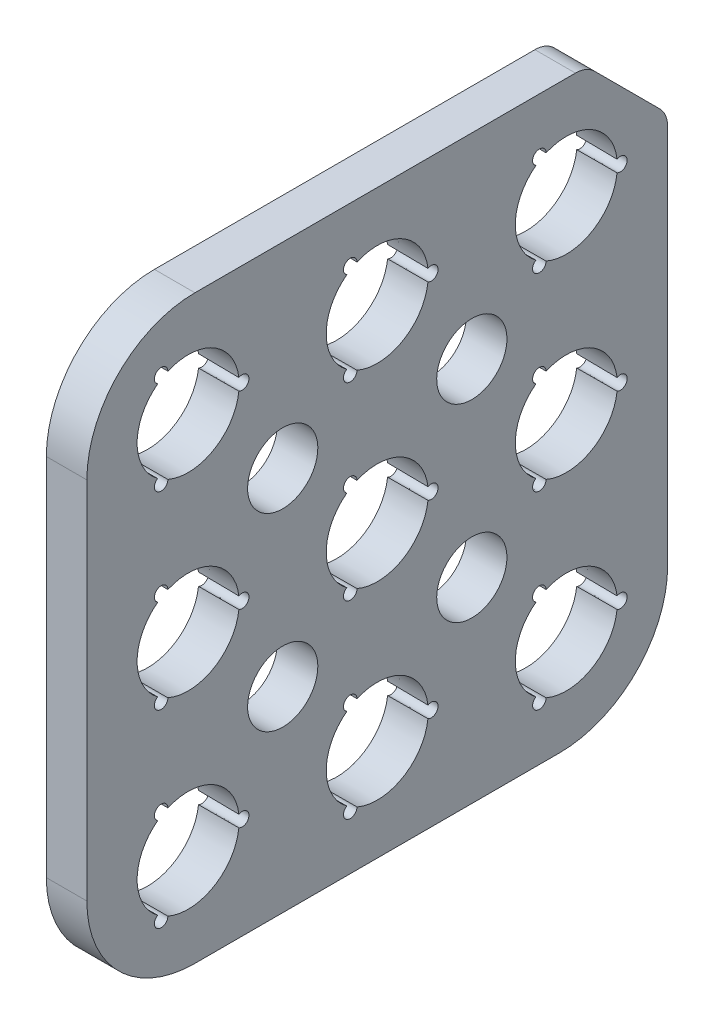
from build123d import *

# Parameters (mm, degrees)
SKETCH_1_W                        = 230
SKETCH_1_H                        = 230
EXTRUDE_1_DEPTH                   = 12.5
SKETCH_6_R                        = 2.475
CUT_EXTRUDE_1_DEPTH               = 47
CUT_EXTRUDE_1_DRAFT               = -0.3
CUT_EXTRUDE_1_PROFILE_2_DEPTH     = 47
CUT_EXTRUDE_1_PROFILE_2_DRAFT     = -0.3
CUT_EXTRUDE_1_PROFILE_3_DEPTH     = 47
CUT_EXTRUDE_1_PROFILE_3_DRAFT     = -0.3
CUT_EXTRUDE_2_DEPTH               = 4
PATTERN_LINEAR_3_COUNT            = 3
PATTERN_LINEAR_3_PITCH            = 70
PATTERN_LINEAR_3_COUNT_DIR2       = 3
PATTERN_LINEAR_3_PITCH_DIR2       = 70
PATTERN_LINEAR_3_COPY_1_SKETCH_R  = 2.475
PATTERN_LINEAR_3_COPY_1_DEPTH     = 47
PATTERN_LINEAR_3_COPY_1_DRAFT     = -0.3
PATTERN_LINEAR_3_COPY_2_SKETCH_R  = 2.475
PATTERN_LINEAR_3_COPY_2_DEPTH     = 47
PATTERN_LINEAR_3_COPY_2_DRAFT     = -0.3
PATTERN_LINEAR_3_COPY_3_SKETCH_R  = 2.475
PATTERN_LINEAR_3_COPY_3_DEPTH     = 47
PATTERN_LINEAR_3_COPY_3_DRAFT     = -0.3
PATTERN_LINEAR_3_COPY_4_SKETCH_R  = 2.475
PATTERN_LINEAR_3_COPY_4_DEPTH     = 47
PATTERN_LINEAR_3_COPY_4_DRAFT     = -0.3
PATTERN_LINEAR_3_COPY_5_SKETCH_R  = 2.475
PATTERN_LINEAR_3_COPY_5_DEPTH     = 47
PATTERN_LINEAR_3_COPY_5_DRAFT     = -0.3
PATTERN_LINEAR_3_COPY_6_SKETCH_R  = 2.475
PATTERN_LINEAR_3_COPY_6_DEPTH     = 47
PATTERN_LINEAR_3_COPY_6_DRAFT     = -0.3
PATTERN_LINEAR_3_COPY_7_SKETCH_R  = 2.475
PATTERN_LINEAR_3_COPY_7_DEPTH     = 47
PATTERN_LINEAR_3_COPY_7_DRAFT     = -0.3
PATTERN_LINEAR_3_COPY_8_SKETCH_R  = 2.475
PATTERN_LINEAR_3_COPY_8_DEPTH     = 47
PATTERN_LINEAR_3_COPY_8_DRAFT     = -0.3
PATTERN_LINEAR_3_COPY_9_SKETCH_R  = 2.475
PATTERN_LINEAR_3_COPY_9_DEPTH     = 47
PATTERN_LINEAR_3_COPY_9_DRAFT     = -0.3
PATTERN_LINEAR_3_COPY_10_SKETCH_R = 2.475
PATTERN_LINEAR_3_COPY_10_DEPTH    = 47
PATTERN_LINEAR_3_COPY_10_DRAFT    = -0.3
PATTERN_LINEAR_3_COPY_11_SKETCH_R = 2.475
PATTERN_LINEAR_3_COPY_11_DEPTH    = 47
PATTERN_LINEAR_3_COPY_11_DRAFT    = -0.3
PATTERN_LINEAR_3_COPY_12_SKETCH_R = 2.475
PATTERN_LINEAR_3_COPY_12_DEPTH    = 47
PATTERN_LINEAR_3_COPY_12_DRAFT    = -0.3
PATTERN_LINEAR_3_COPY_13_SKETCH_R = 2.475
PATTERN_LINEAR_3_COPY_13_DEPTH    = 47
PATTERN_LINEAR_3_COPY_13_DRAFT    = -0.3
PATTERN_LINEAR_3_COPY_14_SKETCH_R = 2.475
PATTERN_LINEAR_3_COPY_14_DEPTH    = 47
PATTERN_LINEAR_3_COPY_14_DRAFT    = -0.3
PATTERN_LINEAR_3_COPY_15_SKETCH_R = 2.475
PATTERN_LINEAR_3_COPY_15_DEPTH    = 47
PATTERN_LINEAR_3_COPY_15_DRAFT    = -0.3
PATTERN_LINEAR_3_COPY_16_SKETCH_R = 2.475
PATTERN_LINEAR_3_COPY_16_DEPTH    = 47
PATTERN_LINEAR_3_COPY_16_DRAFT    = -0.3
PATTERN_LINEAR_3_COPY_17_SKETCH_R = 2.475
PATTERN_LINEAR_3_COPY_17_DEPTH    = 47
PATTERN_LINEAR_3_COPY_17_DRAFT    = -0.3
PATTERN_LINEAR_3_COPY_18_SKETCH_R = 2.475
PATTERN_LINEAR_3_COPY_18_DEPTH    = 47
PATTERN_LINEAR_3_COPY_18_DRAFT    = -0.3
PATTERN_LINEAR_3_COPY_19_SKETCH_R = 2.475
PATTERN_LINEAR_3_COPY_19_DEPTH    = 47
PATTERN_LINEAR_3_COPY_19_DRAFT    = -0.3
PATTERN_LINEAR_3_COPY_20_SKETCH_R = 2.475
PATTERN_LINEAR_3_COPY_20_DEPTH    = 47
PATTERN_LINEAR_3_COPY_20_DRAFT    = -0.3
PATTERN_LINEAR_3_COPY_21_SKETCH_R = 2.475
PATTERN_LINEAR_3_COPY_21_DEPTH    = 47
PATTERN_LINEAR_3_COPY_21_DRAFT    = -0.3
PATTERN_LINEAR_3_COPY_22_SKETCH_R = 2.475
PATTERN_LINEAR_3_COPY_22_DEPTH    = 47
PATTERN_LINEAR_3_COPY_22_DRAFT    = -0.3
PATTERN_LINEAR_3_COPY_23_SKETCH_R = 2.475
PATTERN_LINEAR_3_COPY_23_DEPTH    = 47
PATTERN_LINEAR_3_COPY_23_DRAFT    = -0.3
PATTERN_LINEAR_3_COPY_24_SKETCH_R = 2.475
PATTERN_LINEAR_3_COPY_24_DEPTH    = 47
PATTERN_LINEAR_3_COPY_24_DRAFT    = -0.3
PATTERN_LINEAR_3_COPY_25_SKETCH_R = 2.475
PATTERN_LINEAR_3_COPY_25_DEPTH    = 47
PATTERN_LINEAR_3_COPY_25_DRAFT    = -0.3
PATTERN_LINEAR_3_COPY_26_SKETCH_R = 2.475
PATTERN_LINEAR_3_COPY_26_DEPTH    = 47
PATTERN_LINEAR_3_COPY_26_DRAFT    = -0.3
PATTERN_LINEAR_3_COPY_27_SKETCH_R = 2.475
PATTERN_LINEAR_3_COPY_27_DEPTH    = 47
PATTERN_LINEAR_3_COPY_27_DRAFT    = -0.3
PATTERN_LINEAR_3_COPY_28_SKETCH_R = 2.475
PATTERN_LINEAR_3_COPY_28_DEPTH    = 47
PATTERN_LINEAR_3_COPY_28_DRAFT    = -0.3
PATTERN_LINEAR_3_COPY_29_SKETCH_R = 2.475
PATTERN_LINEAR_3_COPY_29_DEPTH    = 47
PATTERN_LINEAR_3_COPY_29_DRAFT    = -0.3
PATTERN_LINEAR_3_COPY_30_SKETCH_R = 2.475
PATTERN_LINEAR_3_COPY_30_DEPTH    = 47
PATTERN_LINEAR_3_COPY_30_DRAFT    = -0.3
PATTERN_LINEAR_3_COPY_31_SKETCH_R = 2.475
PATTERN_LINEAR_3_COPY_31_DEPTH    = 47
PATTERN_LINEAR_3_COPY_31_DRAFT    = -0.3
PATTERN_LINEAR_3_COPY_32_SKETCH_R = 2.475
PATTERN_LINEAR_3_COPY_32_DEPTH    = 47
PATTERN_LINEAR_3_COPY_32_DRAFT    = -0.3
PATTERN_LINEAR_3_COPY_33_SKETCH_R = 2.475
PATTERN_LINEAR_3_COPY_33_DEPTH    = 47
PATTERN_LINEAR_3_COPY_33_DRAFT    = -0.3
PATTERN_LINEAR_3_COPY_34_SKETCH_R = 2.475
PATTERN_LINEAR_3_COPY_34_DEPTH    = 47
PATTERN_LINEAR_3_COPY_34_DRAFT    = -0.3
PATTERN_LINEAR_3_COPY_35_SKETCH_R = 2.475
PATTERN_LINEAR_3_COPY_35_DEPTH    = 47
PATTERN_LINEAR_3_COPY_35_DRAFT    = -0.3
PATTERN_LINEAR_3_COPY_36_SKETCH_R = 2.475
PATTERN_LINEAR_3_COPY_36_DEPTH    = 47
PATTERN_LINEAR_3_COPY_36_DRAFT    = -0.3
PATTERN_LINEAR_3_COPY_37_SKETCH_R = 2.475
PATTERN_LINEAR_3_COPY_37_DEPTH    = 47
PATTERN_LINEAR_3_COPY_37_DRAFT    = -0.3
PATTERN_LINEAR_3_COPY_38_SKETCH_R = 2.475
PATTERN_LINEAR_3_COPY_38_DEPTH    = 47
PATTERN_LINEAR_3_COPY_38_DRAFT    = -0.3
PATTERN_LINEAR_3_COPY_39_SKETCH_R = 2.475
PATTERN_LINEAR_3_COPY_39_DEPTH    = 47
PATTERN_LINEAR_3_COPY_39_DRAFT    = -0.3
PATTERN_LINEAR_3_COPY_40_SKETCH_R = 2.475
PATTERN_LINEAR_3_COPY_40_DEPTH    = 47
PATTERN_LINEAR_3_COPY_40_DRAFT    = -0.3
SKETCH_8_W                        = 34.590931249
SKETCH_8_H                        = 260.535950259
CUT_EXTRUDE_3_DEPTH               = 626
SKETCH_9_W                        = 249.849241437
SKETCH_9_H                        = 239.022710494
CUT_EXTRUDE_4_DEPTH               = 626
SKETCH_10_W                       = 30.276924454
SKETCH_10_H                       = 249.230780566
CUT_EXTRUDE_5_DEPTH               = 313
SKETCH_11_W                       = 446.10197795
SKETCH_11_H                       = 340.76642687
SKETCH_11_W_2                     = 215
SKETCH_11_H_2                     = 215
CUT_EXTRUDE_6_DEPTH               = 120
CHAMFER_1_SIZE                    = 30
FILLET_1_R                        = 10
FILLET_2_R                        = 40
SKETCH_14_R                       = 13
CUT_EXTRUDE_7_DEPTH               = 120
PATTERN_LINEAR_6_COUNT            = 2
PATTERN_LINEAR_6_PITCH            = 70
PATTERN_LINEAR_6_COUNT_DIR2       = 2
PATTERN_LINEAR_6_PITCH_DIR2       = 70


with BuildPart() as part:
    # 草图1 → 凸台-拉伸1 (new, symmetric)
    with BuildSketch(Plane(origin=(0, 0, 0), x_dir=(0, 0, -1), z_dir=(1, 0, 0))):
        Rectangle(SKETCH_1_W, SKETCH_1_H)
    extrude(amount=EXTRUDE_1_DEPTH, both=True)

    # 草图5 → 切除-旋转1 (revolve, cut)
    with BuildSketch(Plane(origin=(0, 70, 0), x_dir=(1, 0, 0), z_dir=(0, 1, 0))):
        Polygon((9.1, 70), (9.1, 88.87), (-16.76003836, 89.005404082), (-16.76003836, 70), align=None)
    cut_revolve_1 = revolve(axis=Axis((12.711537601, 70, -70), (-1, 0, 0)), mode=Mode.SUBTRACT)


with BuildPart() as cut_extrude_1_tool:
    # 草图6 → 切除-拉伸1 (with draft: the straight prism first)
    with BuildSketch(Plane.ZY.offset(-9.1)):
        with Locations((-60, 87.320508076)):
            Circle(SKETCH_6_R)
    extrude(amount=CUT_EXTRUDE_1_DEPTH)
    # 切除-拉伸1: the draft: its side faces are tilted about the plane it starts from
    cut_extrude_1_sides = [cut_extrude_1_tool.faces().sort_by_distance(p)[0] for p in [
        (-14.4, 87.320508076, -62.475),
    ]]
    draft(cut_extrude_1_sides, Plane.ZY.offset(-9.1), CUT_EXTRUDE_1_DRAFT)


with BuildPart() as part_1:
    add(part.part)

    # 切除-拉伸1: cut by cut_extrude_1_tool
    add(cut_extrude_1_tool.part, mode=Mode.SUBTRACT)


with BuildPart() as cut_extrude_1_profile_2_tool:
    # 草图6 → 切除-拉伸1 profile 2 (with draft: the straight prism first)
    with BuildSketch(Plane.ZY.offset(-9.1)):
        with Locations((-60, 52.679491924)):
            Circle(SKETCH_6_R)
    extrude(amount=CUT_EXTRUDE_1_PROFILE_2_DEPTH)
    # 切除-拉伸1 profile 2: the draft: its side faces are tilted about the plane it starts from
    cut_extrude_1_profile_2_sides = [cut_extrude_1_profile_2_tool.faces().sort_by_distance(p)[0] for p in [
        (-14.4, 52.679491924, -62.475),
    ]]
    draft(cut_extrude_1_profile_2_sides, Plane.ZY.offset(-9.1), CUT_EXTRUDE_1_PROFILE_2_DRAFT)


with BuildPart() as part_2:
    add(part_1.part)

    # 切除-拉伸1 profile 2: cut by cut_extrude_1_profile_2_tool
    add(cut_extrude_1_profile_2_tool.part, mode=Mode.SUBTRACT)


with BuildPart() as cut_extrude_1_profile_3_tool:
    # 草图6 → 切除-拉伸1 profile 3 (with draft: the straight prism first)
    with BuildSketch(Plane.ZY.offset(-9.1)):
        with Locations((-90, 70)):
            Circle(SKETCH_6_R)
    extrude(amount=CUT_EXTRUDE_1_PROFILE_3_DEPTH)
    # 切除-拉伸1 profile 3: the draft: its side faces are tilted about the plane it starts from
    cut_extrude_1_profile_3_sides = [cut_extrude_1_profile_3_tool.faces().sort_by_distance(p)[0] for p in [
        (-14.4, 70, -92.475),
    ]]
    draft(cut_extrude_1_profile_3_sides, Plane.ZY.offset(-9.1), CUT_EXTRUDE_1_PROFILE_3_DRAFT)


with BuildPart() as part_3:
    add(part_2.part)

    # 切除-拉伸1 profile 3: cut by cut_extrude_1_profile_3_tool
    add(cut_extrude_1_profile_3_tool.part, mode=Mode.SUBTRACT)

    # 草图7 → 切除-拉伸2 (cut)
    with BuildSketch(Plane.ZY.offset(12.5)):
        with BuildLine():
            Line((-80.578681475, 81.195601737), (-84.104368777, 87.242876251))
            ThreePointArc((-84.104368777, 87.242876251), (-82.843575171, 92.029357159), (-78.057094263, 90.768563553))
            Line((-78.057094263, 90.768563553), (-74.531406961, 84.721289038))
            ThreePointArc((-74.531406961, 84.721289038), (-75.792200567, 79.934808131), (-80.578681475, 81.195601737))
        make_face()
        with BuildLine():
            Line((-73.5, 85), (-73.5, 92))
            ThreePointArc((-73.5, 92), (-70, 95.5), (-66.5, 92))
            Line((-66.5, 92), (-66.5, 85))
            ThreePointArc((-66.5, 85), (-70, 81.5), (-73.5, 85))
        make_face()
    cut_extrude_2 = extrude(amount=-CUT_EXTRUDE_2_DEPTH, mode=Mode.SUBTRACT)

    # 阵列(线性)3: 切除-旋转1, Cut-Extrude 2 3 × 3
    with Locations(*[(0, -j * PATTERN_LINEAR_3_PITCH_DIR2, i * PATTERN_LINEAR_3_PITCH) for i in range(PATTERN_LINEAR_3_COUNT) for j in range(PATTERN_LINEAR_3_COUNT_DIR2) if (i, j) != (0, 0)]):
        add(cut_revolve_1, mode=Mode.SUBTRACT)
        add(cut_extrude_2, mode=Mode.SUBTRACT)


with BuildPart() as pattern_linear_3_copy_1_tool:
    # 阵列(线性)3 copy 1 sketch → 阵列(线性)3 copy 1 (with draft: the straight prism first)
    with BuildSketch(Plane(origin=(9.1, -70, 0), x_dir=(0, 0, 1), z_dir=(-1, 0, 0))):
        with Locations((-60, 87.320508076)):
            Circle(PATTERN_LINEAR_3_COPY_1_SKETCH_R)
    extrude(amount=PATTERN_LINEAR_3_COPY_1_DEPTH)
    # 阵列(线性)3 copy 1: the draft: its side faces are tilted about the plane it starts from
    pattern_linear_3_copy_1_sides = [pattern_linear_3_copy_1_tool.faces().sort_by_distance(p)[0] for p in [
        (-14.4, 17.320508076, -62.475),
    ]]
    draft(pattern_linear_3_copy_1_sides, Plane(origin=(9.1, -70, 0), x_dir=(0, 0, 1), z_dir=(-1, 0, 0)), PATTERN_LINEAR_3_COPY_1_DRAFT)


with BuildPart() as part_4:
    add(part_3.part)

    # 阵列(线性)3 copy 1: cut by pattern_linear_3_copy_1_tool
    add(pattern_linear_3_copy_1_tool.part, mode=Mode.SUBTRACT)


with BuildPart() as pattern_linear_3_copy_2_tool:
    # 阵列(线性)3 copy 2 sketch → 阵列(线性)3 copy 2 (with draft: the straight prism first)
    with BuildSketch(Plane(origin=(9.1, -140, 0), x_dir=(0, 0, 1), z_dir=(-1, 0, 0))):
        with Locations((-60, 87.320508076)):
            Circle(PATTERN_LINEAR_3_COPY_2_SKETCH_R)
    extrude(amount=PATTERN_LINEAR_3_COPY_2_DEPTH)
    # 阵列(线性)3 copy 2: the draft: its side faces are tilted about the plane it starts from
    pattern_linear_3_copy_2_sides = [pattern_linear_3_copy_2_tool.faces().sort_by_distance(p)[0] for p in [
        (-14.4, -52.679491924, -62.475),
    ]]
    draft(pattern_linear_3_copy_2_sides, Plane(origin=(9.1, -140, 0), x_dir=(0, 0, 1), z_dir=(-1, 0, 0)), PATTERN_LINEAR_3_COPY_2_DRAFT)


with BuildPart() as part_5:
    add(part_4.part)

    # 阵列(线性)3 copy 2: cut by pattern_linear_3_copy_2_tool
    add(pattern_linear_3_copy_2_tool.part, mode=Mode.SUBTRACT)


with BuildPart() as pattern_linear_3_copy_3_tool:
    # 阵列(线性)3 copy 3 sketch → 阵列(线性)3 copy 3 (with draft: the straight prism first)
    with BuildSketch(Plane(origin=(9.1, 0, 70), x_dir=(0, 0, 1), z_dir=(-1, 0, 0))):
        with Locations((-60, 87.320508076)):
            Circle(PATTERN_LINEAR_3_COPY_3_SKETCH_R)
    extrude(amount=PATTERN_LINEAR_3_COPY_3_DEPTH)
    # 阵列(线性)3 copy 3: the draft: its side faces are tilted about the plane it starts from
    pattern_linear_3_copy_3_sides = [pattern_linear_3_copy_3_tool.faces().sort_by_distance(p)[0] for p in [
        (-14.4, 87.320508076, 7.525),
    ]]
    draft(pattern_linear_3_copy_3_sides, Plane(origin=(9.1, 0, 70), x_dir=(0, 0, 1), z_dir=(-1, 0, 0)), PATTERN_LINEAR_3_COPY_3_DRAFT)


with BuildPart() as part_6:
    add(part_5.part)

    # 阵列(线性)3 copy 3: cut by pattern_linear_3_copy_3_tool
    add(pattern_linear_3_copy_3_tool.part, mode=Mode.SUBTRACT)


with BuildPart() as pattern_linear_3_copy_4_tool:
    # 阵列(线性)3 copy 4 sketch → 阵列(线性)3 copy 4 (with draft: the straight prism first)
    with BuildSketch(Plane(origin=(9.1, -70, 70), x_dir=(0, 0, 1), z_dir=(-1, 0, 0))):
        with Locations((-60, 87.320508076)):
            Circle(PATTERN_LINEAR_3_COPY_4_SKETCH_R)
    extrude(amount=PATTERN_LINEAR_3_COPY_4_DEPTH)
    # 阵列(线性)3 copy 4: the draft: its side faces are tilted about the plane it starts from
    pattern_linear_3_copy_4_sides = [pattern_linear_3_copy_4_tool.faces().sort_by_distance(p)[0] for p in [
        (-14.4, 17.320508076, 7.525),
    ]]
    draft(pattern_linear_3_copy_4_sides, Plane(origin=(9.1, -70, 70), x_dir=(0, 0, 1), z_dir=(-1, 0, 0)), PATTERN_LINEAR_3_COPY_4_DRAFT)


with BuildPart() as part_7:
    add(part_6.part)

    # 阵列(线性)3 copy 4: cut by pattern_linear_3_copy_4_tool
    add(pattern_linear_3_copy_4_tool.part, mode=Mode.SUBTRACT)


with BuildPart() as pattern_linear_3_copy_5_tool:
    # 阵列(线性)3 copy 5 sketch → 阵列(线性)3 copy 5 (with draft: the straight prism first)
    with BuildSketch(Plane(origin=(9.1, -140, 70), x_dir=(0, 0, 1), z_dir=(-1, 0, 0))):
        with Locations((-60, 87.320508076)):
            Circle(PATTERN_LINEAR_3_COPY_5_SKETCH_R)
    extrude(amount=PATTERN_LINEAR_3_COPY_5_DEPTH)
    # 阵列(线性)3 copy 5: the draft: its side faces are tilted about the plane it starts from
    pattern_linear_3_copy_5_sides = [pattern_linear_3_copy_5_tool.faces().sort_by_distance(p)[0] for p in [
        (-14.4, -52.679491924, 7.525),
    ]]
    draft(pattern_linear_3_copy_5_sides, Plane(origin=(9.1, -140, 70), x_dir=(0, 0, 1), z_dir=(-1, 0, 0)), PATTERN_LINEAR_3_COPY_5_DRAFT)


with BuildPart() as part_8:
    add(part_7.part)

    # 阵列(线性)3 copy 5: cut by pattern_linear_3_copy_5_tool
    add(pattern_linear_3_copy_5_tool.part, mode=Mode.SUBTRACT)


with BuildPart() as pattern_linear_3_copy_6_tool:
    # 阵列(线性)3 copy 6 sketch → 阵列(线性)3 copy 6 (with draft: the straight prism first)
    with BuildSketch(Plane(origin=(9.1, 0, 140), x_dir=(0, 0, 1), z_dir=(-1, 0, 0))):
        with Locations((-60, 87.320508076)):
            Circle(PATTERN_LINEAR_3_COPY_6_SKETCH_R)
    extrude(amount=PATTERN_LINEAR_3_COPY_6_DEPTH)
    # 阵列(线性)3 copy 6: the draft: its side faces are tilted about the plane it starts from
    pattern_linear_3_copy_6_sides = [pattern_linear_3_copy_6_tool.faces().sort_by_distance(p)[0] for p in [
        (-14.4, 87.320508076, 77.525),
    ]]
    draft(pattern_linear_3_copy_6_sides, Plane(origin=(9.1, 0, 140), x_dir=(0, 0, 1), z_dir=(-1, 0, 0)), PATTERN_LINEAR_3_COPY_6_DRAFT)


with BuildPart() as part_9:
    add(part_8.part)

    # 阵列(线性)3 copy 6: cut by pattern_linear_3_copy_6_tool
    add(pattern_linear_3_copy_6_tool.part, mode=Mode.SUBTRACT)


with BuildPart() as pattern_linear_3_copy_7_tool:
    # 阵列(线性)3 copy 7 sketch → 阵列(线性)3 copy 7 (with draft: the straight prism first)
    with BuildSketch(Plane(origin=(9.1, -70, 140), x_dir=(0, 0, 1), z_dir=(-1, 0, 0))):
        with Locations((-60, 87.320508076)):
            Circle(PATTERN_LINEAR_3_COPY_7_SKETCH_R)
    extrude(amount=PATTERN_LINEAR_3_COPY_7_DEPTH)
    # 阵列(线性)3 copy 7: the draft: its side faces are tilted about the plane it starts from
    pattern_linear_3_copy_7_sides = [pattern_linear_3_copy_7_tool.faces().sort_by_distance(p)[0] for p in [
        (-14.4, 17.320508076, 77.525),
    ]]
    draft(pattern_linear_3_copy_7_sides, Plane(origin=(9.1, -70, 140), x_dir=(0, 0, 1), z_dir=(-1, 0, 0)), PATTERN_LINEAR_3_COPY_7_DRAFT)


with BuildPart() as part_10:
    add(part_9.part)

    # 阵列(线性)3 copy 7: cut by pattern_linear_3_copy_7_tool
    add(pattern_linear_3_copy_7_tool.part, mode=Mode.SUBTRACT)


with BuildPart() as pattern_linear_3_copy_8_tool:
    # 阵列(线性)3 copy 8 sketch → 阵列(线性)3 copy 8 (with draft: the straight prism first)
    with BuildSketch(Plane(origin=(9.1, -140, 140), x_dir=(0, 0, 1), z_dir=(-1, 0, 0))):
        with Locations((-60, 87.320508076)):
            Circle(PATTERN_LINEAR_3_COPY_8_SKETCH_R)
    extrude(amount=PATTERN_LINEAR_3_COPY_8_DEPTH)
    # 阵列(线性)3 copy 8: the draft: its side faces are tilted about the plane it starts from
    pattern_linear_3_copy_8_sides = [pattern_linear_3_copy_8_tool.faces().sort_by_distance(p)[0] for p in [
        (-14.4, -52.679491924, 77.525),
    ]]
    draft(pattern_linear_3_copy_8_sides, Plane(origin=(9.1, -140, 140), x_dir=(0, 0, 1), z_dir=(-1, 0, 0)), PATTERN_LINEAR_3_COPY_8_DRAFT)


with BuildPart() as part_11:
    add(part_10.part)

    # 阵列(线性)3 copy 8: cut by pattern_linear_3_copy_8_tool
    add(pattern_linear_3_copy_8_tool.part, mode=Mode.SUBTRACT)


with BuildPart() as pattern_linear_3_copy_9_tool:
    # 阵列(线性)3 copy 9 sketch → 阵列(线性)3 copy 9 (with draft: the straight prism first)
    with BuildSketch(Plane(origin=(9.1, -70, 0), x_dir=(0, 0, 1), z_dir=(-1, 0, 0))):
        with Locations((-60, 52.679491924)):
            Circle(PATTERN_LINEAR_3_COPY_9_SKETCH_R)
    extrude(amount=PATTERN_LINEAR_3_COPY_9_DEPTH)
    # 阵列(线性)3 copy 9: the draft: its side faces are tilted about the plane it starts from
    pattern_linear_3_copy_9_sides = [pattern_linear_3_copy_9_tool.faces().sort_by_distance(p)[0] for p in [
        (-14.4, -17.320508076, -62.475),
    ]]
    draft(pattern_linear_3_copy_9_sides, Plane(origin=(9.1, -70, 0), x_dir=(0, 0, 1), z_dir=(-1, 0, 0)), PATTERN_LINEAR_3_COPY_9_DRAFT)


with BuildPart() as part_12:
    add(part_11.part)

    # 阵列(线性)3 copy 9: cut by pattern_linear_3_copy_9_tool
    add(pattern_linear_3_copy_9_tool.part, mode=Mode.SUBTRACT)


with BuildPart() as pattern_linear_3_copy_10_tool:
    # 阵列(线性)3 copy 10 sketch → 阵列(线性)3 copy 10 (with draft: the straight prism first)
    with BuildSketch(Plane(origin=(9.1, -140, 0), x_dir=(0, 0, 1), z_dir=(-1, 0, 0))):
        with Locations((-60, 52.679491924)):
            Circle(PATTERN_LINEAR_3_COPY_10_SKETCH_R)
    extrude(amount=PATTERN_LINEAR_3_COPY_10_DEPTH)
    # 阵列(线性)3 copy 10: the draft: its side faces are tilted about the plane it starts from
    pattern_linear_3_copy_10_sides = [pattern_linear_3_copy_10_tool.faces().sort_by_distance(p)[0] for p in [
        (-14.4, -87.320508076, -62.475),
    ]]
    draft(pattern_linear_3_copy_10_sides, Plane(origin=(9.1, -140, 0), x_dir=(0, 0, 1), z_dir=(-1, 0, 0)), PATTERN_LINEAR_3_COPY_10_DRAFT)


with BuildPart() as part_13:
    add(part_12.part)

    # 阵列(线性)3 copy 10: cut by pattern_linear_3_copy_10_tool
    add(pattern_linear_3_copy_10_tool.part, mode=Mode.SUBTRACT)


with BuildPart() as pattern_linear_3_copy_11_tool:
    # 阵列(线性)3 copy 11 sketch → 阵列(线性)3 copy 11 (with draft: the straight prism first)
    with BuildSketch(Plane(origin=(9.1, 0, 70), x_dir=(0, 0, 1), z_dir=(-1, 0, 0))):
        with Locations((-60, 52.679491924)):
            Circle(PATTERN_LINEAR_3_COPY_11_SKETCH_R)
    extrude(amount=PATTERN_LINEAR_3_COPY_11_DEPTH)
    # 阵列(线性)3 copy 11: the draft: its side faces are tilted about the plane it starts from
    pattern_linear_3_copy_11_sides = [pattern_linear_3_copy_11_tool.faces().sort_by_distance(p)[0] for p in [
        (-14.4, 52.679491924, 7.525),
    ]]
    draft(pattern_linear_3_copy_11_sides, Plane(origin=(9.1, 0, 70), x_dir=(0, 0, 1), z_dir=(-1, 0, 0)), PATTERN_LINEAR_3_COPY_11_DRAFT)


with BuildPart() as part_14:
    add(part_13.part)

    # 阵列(线性)3 copy 11: cut by pattern_linear_3_copy_11_tool
    add(pattern_linear_3_copy_11_tool.part, mode=Mode.SUBTRACT)


with BuildPart() as pattern_linear_3_copy_12_tool:
    # 阵列(线性)3 copy 12 sketch → 阵列(线性)3 copy 12 (with draft: the straight prism first)
    with BuildSketch(Plane(origin=(9.1, -70, 70), x_dir=(0, 0, 1), z_dir=(-1, 0, 0))):
        with Locations((-60, 52.679491924)):
            Circle(PATTERN_LINEAR_3_COPY_12_SKETCH_R)
    extrude(amount=PATTERN_LINEAR_3_COPY_12_DEPTH)
    # 阵列(线性)3 copy 12: the draft: its side faces are tilted about the plane it starts from
    pattern_linear_3_copy_12_sides = [pattern_linear_3_copy_12_tool.faces().sort_by_distance(p)[0] for p in [
        (-14.4, -17.320508076, 7.525),
    ]]
    draft(pattern_linear_3_copy_12_sides, Plane(origin=(9.1, -70, 70), x_dir=(0, 0, 1), z_dir=(-1, 0, 0)), PATTERN_LINEAR_3_COPY_12_DRAFT)


with BuildPart() as part_15:
    add(part_14.part)

    # 阵列(线性)3 copy 12: cut by pattern_linear_3_copy_12_tool
    add(pattern_linear_3_copy_12_tool.part, mode=Mode.SUBTRACT)


with BuildPart() as pattern_linear_3_copy_13_tool:
    # 阵列(线性)3 copy 13 sketch → 阵列(线性)3 copy 13 (with draft: the straight prism first)
    with BuildSketch(Plane(origin=(9.1, -140, 70), x_dir=(0, 0, 1), z_dir=(-1, 0, 0))):
        with Locations((-60, 52.679491924)):
            Circle(PATTERN_LINEAR_3_COPY_13_SKETCH_R)
    extrude(amount=PATTERN_LINEAR_3_COPY_13_DEPTH)
    # 阵列(线性)3 copy 13: the draft: its side faces are tilted about the plane it starts from
    pattern_linear_3_copy_13_sides = [pattern_linear_3_copy_13_tool.faces().sort_by_distance(p)[0] for p in [
        (-14.4, -87.320508076, 7.525),
    ]]
    draft(pattern_linear_3_copy_13_sides, Plane(origin=(9.1, -140, 70), x_dir=(0, 0, 1), z_dir=(-1, 0, 0)), PATTERN_LINEAR_3_COPY_13_DRAFT)


with BuildPart() as part_16:
    add(part_15.part)

    # 阵列(线性)3 copy 13: cut by pattern_linear_3_copy_13_tool
    add(pattern_linear_3_copy_13_tool.part, mode=Mode.SUBTRACT)


with BuildPart() as pattern_linear_3_copy_14_tool:
    # 阵列(线性)3 copy 14 sketch → 阵列(线性)3 copy 14 (with draft: the straight prism first)
    with BuildSketch(Plane(origin=(9.1, 0, 140), x_dir=(0, 0, 1), z_dir=(-1, 0, 0))):
        with Locations((-60, 52.679491924)):
            Circle(PATTERN_LINEAR_3_COPY_14_SKETCH_R)
    extrude(amount=PATTERN_LINEAR_3_COPY_14_DEPTH)
    # 阵列(线性)3 copy 14: the draft: its side faces are tilted about the plane it starts from
    pattern_linear_3_copy_14_sides = [pattern_linear_3_copy_14_tool.faces().sort_by_distance(p)[0] for p in [
        (-14.4, 52.679491924, 77.525),
    ]]
    draft(pattern_linear_3_copy_14_sides, Plane(origin=(9.1, 0, 140), x_dir=(0, 0, 1), z_dir=(-1, 0, 0)), PATTERN_LINEAR_3_COPY_14_DRAFT)


with BuildPart() as part_17:
    add(part_16.part)

    # 阵列(线性)3 copy 14: cut by pattern_linear_3_copy_14_tool
    add(pattern_linear_3_copy_14_tool.part, mode=Mode.SUBTRACT)


with BuildPart() as pattern_linear_3_copy_15_tool:
    # 阵列(线性)3 copy 15 sketch → 阵列(线性)3 copy 15 (with draft: the straight prism first)
    with BuildSketch(Plane(origin=(9.1, -70, 140), x_dir=(0, 0, 1), z_dir=(-1, 0, 0))):
        with Locations((-60, 52.679491924)):
            Circle(PATTERN_LINEAR_3_COPY_15_SKETCH_R)
    extrude(amount=PATTERN_LINEAR_3_COPY_15_DEPTH)
    # 阵列(线性)3 copy 15: the draft: its side faces are tilted about the plane it starts from
    pattern_linear_3_copy_15_sides = [pattern_linear_3_copy_15_tool.faces().sort_by_distance(p)[0] for p in [
        (-14.4, -17.320508076, 77.525),
    ]]
    draft(pattern_linear_3_copy_15_sides, Plane(origin=(9.1, -70, 140), x_dir=(0, 0, 1), z_dir=(-1, 0, 0)), PATTERN_LINEAR_3_COPY_15_DRAFT)


with BuildPart() as part_18:
    add(part_17.part)

    # 阵列(线性)3 copy 15: cut by pattern_linear_3_copy_15_tool
    add(pattern_linear_3_copy_15_tool.part, mode=Mode.SUBTRACT)


with BuildPart() as pattern_linear_3_copy_16_tool:
    # 阵列(线性)3 copy 16 sketch → 阵列(线性)3 copy 16 (with draft: the straight prism first)
    with BuildSketch(Plane(origin=(9.1, -140, 140), x_dir=(0, 0, 1), z_dir=(-1, 0, 0))):
        with Locations((-60, 52.679491924)):
            Circle(PATTERN_LINEAR_3_COPY_16_SKETCH_R)
    extrude(amount=PATTERN_LINEAR_3_COPY_16_DEPTH)
    # 阵列(线性)3 copy 16: the draft: its side faces are tilted about the plane it starts from
    pattern_linear_3_copy_16_sides = [pattern_linear_3_copy_16_tool.faces().sort_by_distance(p)[0] for p in [
        (-14.4, -87.320508076, 77.525),
    ]]
    draft(pattern_linear_3_copy_16_sides, Plane(origin=(9.1, -140, 140), x_dir=(0, 0, 1), z_dir=(-1, 0, 0)), PATTERN_LINEAR_3_COPY_16_DRAFT)


with BuildPart() as part_19:
    add(part_18.part)

    # 阵列(线性)3 copy 16: cut by pattern_linear_3_copy_16_tool
    add(pattern_linear_3_copy_16_tool.part, mode=Mode.SUBTRACT)


with BuildPart() as pattern_linear_3_copy_17_tool:
    # 阵列(线性)3 copy 17 sketch → 阵列(线性)3 copy 17 (with draft: the straight prism first)
    with BuildSketch(Plane(origin=(9.1, -70, 0), x_dir=(0, 0, 1), z_dir=(-1, 0, 0))):
        with Locations((-90, 70)):
            Circle(PATTERN_LINEAR_3_COPY_17_SKETCH_R)
    extrude(amount=PATTERN_LINEAR_3_COPY_17_DEPTH)
    # 阵列(线性)3 copy 17: the draft: its side faces are tilted about the plane it starts from
    pattern_linear_3_copy_17_sides = [pattern_linear_3_copy_17_tool.faces().sort_by_distance(p)[0] for p in [
        (-14.4, 0, -92.475),
    ]]
    draft(pattern_linear_3_copy_17_sides, Plane(origin=(9.1, -70, 0), x_dir=(0, 0, 1), z_dir=(-1, 0, 0)), PATTERN_LINEAR_3_COPY_17_DRAFT)


with BuildPart() as part_20:
    add(part_19.part)

    # 阵列(线性)3 copy 17: cut by pattern_linear_3_copy_17_tool
    add(pattern_linear_3_copy_17_tool.part, mode=Mode.SUBTRACT)


with BuildPart() as pattern_linear_3_copy_18_tool:
    # 阵列(线性)3 copy 18 sketch → 阵列(线性)3 copy 18 (with draft: the straight prism first)
    with BuildSketch(Plane(origin=(9.1, -140, 0), x_dir=(0, 0, 1), z_dir=(-1, 0, 0))):
        with Locations((-90, 70)):
            Circle(PATTERN_LINEAR_3_COPY_18_SKETCH_R)
    extrude(amount=PATTERN_LINEAR_3_COPY_18_DEPTH)
    # 阵列(线性)3 copy 18: the draft: its side faces are tilted about the plane it starts from
    pattern_linear_3_copy_18_sides = [pattern_linear_3_copy_18_tool.faces().sort_by_distance(p)[0] for p in [
        (-14.4, -70, -92.475),
    ]]
    draft(pattern_linear_3_copy_18_sides, Plane(origin=(9.1, -140, 0), x_dir=(0, 0, 1), z_dir=(-1, 0, 0)), PATTERN_LINEAR_3_COPY_18_DRAFT)


with BuildPart() as part_21:
    add(part_20.part)

    # 阵列(线性)3 copy 18: cut by pattern_linear_3_copy_18_tool
    add(pattern_linear_3_copy_18_tool.part, mode=Mode.SUBTRACT)


with BuildPart() as pattern_linear_3_copy_19_tool:
    # 阵列(线性)3 copy 19 sketch → 阵列(线性)3 copy 19 (with draft: the straight prism first)
    with BuildSketch(Plane(origin=(9.1, 0, 70), x_dir=(0, 0, 1), z_dir=(-1, 0, 0))):
        with Locations((-90, 70)):
            Circle(PATTERN_LINEAR_3_COPY_19_SKETCH_R)
    extrude(amount=PATTERN_LINEAR_3_COPY_19_DEPTH)
    # 阵列(线性)3 copy 19: the draft: its side faces are tilted about the plane it starts from
    pattern_linear_3_copy_19_sides = [pattern_linear_3_copy_19_tool.faces().sort_by_distance(p)[0] for p in [
        (-14.4, 70, -22.475),
    ]]
    draft(pattern_linear_3_copy_19_sides, Plane(origin=(9.1, 0, 70), x_dir=(0, 0, 1), z_dir=(-1, 0, 0)), PATTERN_LINEAR_3_COPY_19_DRAFT)


with BuildPart() as part_22:
    add(part_21.part)

    # 阵列(线性)3 copy 19: cut by pattern_linear_3_copy_19_tool
    add(pattern_linear_3_copy_19_tool.part, mode=Mode.SUBTRACT)


with BuildPart() as pattern_linear_3_copy_20_tool:
    # 阵列(线性)3 copy 20 sketch → 阵列(线性)3 copy 20 (with draft: the straight prism first)
    with BuildSketch(Plane(origin=(9.1, -70, 70), x_dir=(0, 0, 1), z_dir=(-1, 0, 0))):
        with Locations((-90, 70)):
            Circle(PATTERN_LINEAR_3_COPY_20_SKETCH_R)
    extrude(amount=PATTERN_LINEAR_3_COPY_20_DEPTH)
    # 阵列(线性)3 copy 20: the draft: its side faces are tilted about the plane it starts from
    pattern_linear_3_copy_20_sides = [pattern_linear_3_copy_20_tool.faces().sort_by_distance(p)[0] for p in [
        (-14.4, 0, -22.475),
    ]]
    draft(pattern_linear_3_copy_20_sides, Plane(origin=(9.1, -70, 70), x_dir=(0, 0, 1), z_dir=(-1, 0, 0)), PATTERN_LINEAR_3_COPY_20_DRAFT)


with BuildPart() as part_23:
    add(part_22.part)

    # 阵列(线性)3 copy 20: cut by pattern_linear_3_copy_20_tool
    add(pattern_linear_3_copy_20_tool.part, mode=Mode.SUBTRACT)


with BuildPart() as pattern_linear_3_copy_21_tool:
    # 阵列(线性)3 copy 21 sketch → 阵列(线性)3 copy 21 (with draft: the straight prism first)
    with BuildSketch(Plane(origin=(9.1, -140, 70), x_dir=(0, 0, 1), z_dir=(-1, 0, 0))):
        with Locations((-90, 70)):
            Circle(PATTERN_LINEAR_3_COPY_21_SKETCH_R)
    extrude(amount=PATTERN_LINEAR_3_COPY_21_DEPTH)
    # 阵列(线性)3 copy 21: the draft: its side faces are tilted about the plane it starts from
    pattern_linear_3_copy_21_sides = [pattern_linear_3_copy_21_tool.faces().sort_by_distance(p)[0] for p in [
        (-14.4, -70, -22.475),
    ]]
    draft(pattern_linear_3_copy_21_sides, Plane(origin=(9.1, -140, 70), x_dir=(0, 0, 1), z_dir=(-1, 0, 0)), PATTERN_LINEAR_3_COPY_21_DRAFT)


with BuildPart() as part_24:
    add(part_23.part)

    # 阵列(线性)3 copy 21: cut by pattern_linear_3_copy_21_tool
    add(pattern_linear_3_copy_21_tool.part, mode=Mode.SUBTRACT)


with BuildPart() as pattern_linear_3_copy_22_tool:
    # 阵列(线性)3 copy 22 sketch → 阵列(线性)3 copy 22 (with draft: the straight prism first)
    with BuildSketch(Plane(origin=(9.1, 0, 140), x_dir=(0, 0, 1), z_dir=(-1, 0, 0))):
        with Locations((-90, 70)):
            Circle(PATTERN_LINEAR_3_COPY_22_SKETCH_R)
    extrude(amount=PATTERN_LINEAR_3_COPY_22_DEPTH)
    # 阵列(线性)3 copy 22: the draft: its side faces are tilted about the plane it starts from
    pattern_linear_3_copy_22_sides = [pattern_linear_3_copy_22_tool.faces().sort_by_distance(p)[0] for p in [
        (-14.4, 70, 47.525),
    ]]
    draft(pattern_linear_3_copy_22_sides, Plane(origin=(9.1, 0, 140), x_dir=(0, 0, 1), z_dir=(-1, 0, 0)), PATTERN_LINEAR_3_COPY_22_DRAFT)


with BuildPart() as part_25:
    add(part_24.part)

    # 阵列(线性)3 copy 22: cut by pattern_linear_3_copy_22_tool
    add(pattern_linear_3_copy_22_tool.part, mode=Mode.SUBTRACT)


with BuildPart() as pattern_linear_3_copy_23_tool:
    # 阵列(线性)3 copy 23 sketch → 阵列(线性)3 copy 23 (with draft: the straight prism first)
    with BuildSketch(Plane(origin=(9.1, -70, 140), x_dir=(0, 0, 1), z_dir=(-1, 0, 0))):
        with Locations((-90, 70)):
            Circle(PATTERN_LINEAR_3_COPY_23_SKETCH_R)
    extrude(amount=PATTERN_LINEAR_3_COPY_23_DEPTH)
    # 阵列(线性)3 copy 23: the draft: its side faces are tilted about the plane it starts from
    pattern_linear_3_copy_23_sides = [pattern_linear_3_copy_23_tool.faces().sort_by_distance(p)[0] for p in [
        (-14.4, 0, 47.525),
    ]]
    draft(pattern_linear_3_copy_23_sides, Plane(origin=(9.1, -70, 140), x_dir=(0, 0, 1), z_dir=(-1, 0, 0)), PATTERN_LINEAR_3_COPY_23_DRAFT)


with BuildPart() as part_26:
    add(part_25.part)

    # 阵列(线性)3 copy 23: cut by pattern_linear_3_copy_23_tool
    add(pattern_linear_3_copy_23_tool.part, mode=Mode.SUBTRACT)


with BuildPart() as pattern_linear_3_copy_24_tool:
    # 阵列(线性)3 copy 24 sketch → 阵列(线性)3 copy 24 (with draft: the straight prism first)
    with BuildSketch(Plane(origin=(9.1, -140, 140), x_dir=(0, 0, 1), z_dir=(-1, 0, 0))):
        with Locations((-90, 70)):
            Circle(PATTERN_LINEAR_3_COPY_24_SKETCH_R)
    extrude(amount=PATTERN_LINEAR_3_COPY_24_DEPTH)
    # 阵列(线性)3 copy 24: the draft: its side faces are tilted about the plane it starts from
    pattern_linear_3_copy_24_sides = [pattern_linear_3_copy_24_tool.faces().sort_by_distance(p)[0] for p in [
        (-14.4, -70, 47.525),
    ]]
    draft(pattern_linear_3_copy_24_sides, Plane(origin=(9.1, -140, 140), x_dir=(0, 0, 1), z_dir=(-1, 0, 0)), PATTERN_LINEAR_3_COPY_24_DRAFT)


with BuildPart() as part_27:
    add(part_26.part)

    # 阵列(线性)3 copy 24: cut by pattern_linear_3_copy_24_tool
    add(pattern_linear_3_copy_24_tool.part, mode=Mode.SUBTRACT)


with BuildPart() as pattern_linear_3_copy_25_tool:
    # 阵列(线性)3 copy 25 sketch → 阵列(线性)3 copy 25 (with draft: the straight prism first)
    with BuildSketch(Plane(origin=(9.1, -70, 0), x_dir=(0, 0, 1), z_dir=(-1, 0, 0))):
        with Locations((-60, 52.679491924)):
            Circle(PATTERN_LINEAR_3_COPY_25_SKETCH_R)
    extrude(amount=PATTERN_LINEAR_3_COPY_25_DEPTH)
    # 阵列(线性)3 copy 25: the draft: its side faces are tilted about the plane it starts from
    pattern_linear_3_copy_25_sides = [pattern_linear_3_copy_25_tool.faces().sort_by_distance(p)[0] for p in [
        (-14.4, -17.320508076, -62.475),
    ]]
    draft(pattern_linear_3_copy_25_sides, Plane(origin=(9.1, -70, 0), x_dir=(0, 0, 1), z_dir=(-1, 0, 0)), PATTERN_LINEAR_3_COPY_25_DRAFT)


with BuildPart() as part_28:
    add(part_27.part)

    # 阵列(线性)3 copy 25: cut by pattern_linear_3_copy_25_tool
    add(pattern_linear_3_copy_25_tool.part, mode=Mode.SUBTRACT)


with BuildPart() as pattern_linear_3_copy_26_tool:
    # 阵列(线性)3 copy 26 sketch → 阵列(线性)3 copy 26 (with draft: the straight prism first)
    with BuildSketch(Plane(origin=(9.1, -140, 0), x_dir=(0, 0, 1), z_dir=(-1, 0, 0))):
        with Locations((-60, 52.679491924)):
            Circle(PATTERN_LINEAR_3_COPY_26_SKETCH_R)
    extrude(amount=PATTERN_LINEAR_3_COPY_26_DEPTH)
    # 阵列(线性)3 copy 26: the draft: its side faces are tilted about the plane it starts from
    pattern_linear_3_copy_26_sides = [pattern_linear_3_copy_26_tool.faces().sort_by_distance(p)[0] for p in [
        (-14.4, -87.320508076, -62.475),
    ]]
    draft(pattern_linear_3_copy_26_sides, Plane(origin=(9.1, -140, 0), x_dir=(0, 0, 1), z_dir=(-1, 0, 0)), PATTERN_LINEAR_3_COPY_26_DRAFT)


with BuildPart() as part_29:
    add(part_28.part)

    # 阵列(线性)3 copy 26: cut by pattern_linear_3_copy_26_tool
    add(pattern_linear_3_copy_26_tool.part, mode=Mode.SUBTRACT)


with BuildPart() as pattern_linear_3_copy_27_tool:
    # 阵列(线性)3 copy 27 sketch → 阵列(线性)3 copy 27 (with draft: the straight prism first)
    with BuildSketch(Plane(origin=(9.1, 0, 70), x_dir=(0, 0, 1), z_dir=(-1, 0, 0))):
        with Locations((-60, 52.679491924)):
            Circle(PATTERN_LINEAR_3_COPY_27_SKETCH_R)
    extrude(amount=PATTERN_LINEAR_3_COPY_27_DEPTH)
    # 阵列(线性)3 copy 27: the draft: its side faces are tilted about the plane it starts from
    pattern_linear_3_copy_27_sides = [pattern_linear_3_copy_27_tool.faces().sort_by_distance(p)[0] for p in [
        (-14.4, 52.679491924, 7.525),
    ]]
    draft(pattern_linear_3_copy_27_sides, Plane(origin=(9.1, 0, 70), x_dir=(0, 0, 1), z_dir=(-1, 0, 0)), PATTERN_LINEAR_3_COPY_27_DRAFT)


with BuildPart() as part_30:
    add(part_29.part)

    # 阵列(线性)3 copy 27: cut by pattern_linear_3_copy_27_tool
    add(pattern_linear_3_copy_27_tool.part, mode=Mode.SUBTRACT)


with BuildPart() as pattern_linear_3_copy_28_tool:
    # 阵列(线性)3 copy 28 sketch → 阵列(线性)3 copy 28 (with draft: the straight prism first)
    with BuildSketch(Plane(origin=(9.1, -70, 70), x_dir=(0, 0, 1), z_dir=(-1, 0, 0))):
        with Locations((-60, 52.679491924)):
            Circle(PATTERN_LINEAR_3_COPY_28_SKETCH_R)
    extrude(amount=PATTERN_LINEAR_3_COPY_28_DEPTH)
    # 阵列(线性)3 copy 28: the draft: its side faces are tilted about the plane it starts from
    pattern_linear_3_copy_28_sides = [pattern_linear_3_copy_28_tool.faces().sort_by_distance(p)[0] for p in [
        (-14.4, -17.320508076, 7.525),
    ]]
    draft(pattern_linear_3_copy_28_sides, Plane(origin=(9.1, -70, 70), x_dir=(0, 0, 1), z_dir=(-1, 0, 0)), PATTERN_LINEAR_3_COPY_28_DRAFT)


with BuildPart() as part_31:
    add(part_30.part)

    # 阵列(线性)3 copy 28: cut by pattern_linear_3_copy_28_tool
    add(pattern_linear_3_copy_28_tool.part, mode=Mode.SUBTRACT)


with BuildPart() as pattern_linear_3_copy_29_tool:
    # 阵列(线性)3 copy 29 sketch → 阵列(线性)3 copy 29 (with draft: the straight prism first)
    with BuildSketch(Plane(origin=(9.1, -140, 70), x_dir=(0, 0, 1), z_dir=(-1, 0, 0))):
        with Locations((-60, 52.679491924)):
            Circle(PATTERN_LINEAR_3_COPY_29_SKETCH_R)
    extrude(amount=PATTERN_LINEAR_3_COPY_29_DEPTH)
    # 阵列(线性)3 copy 29: the draft: its side faces are tilted about the plane it starts from
    pattern_linear_3_copy_29_sides = [pattern_linear_3_copy_29_tool.faces().sort_by_distance(p)[0] for p in [
        (-14.4, -87.320508076, 7.525),
    ]]
    draft(pattern_linear_3_copy_29_sides, Plane(origin=(9.1, -140, 70), x_dir=(0, 0, 1), z_dir=(-1, 0, 0)), PATTERN_LINEAR_3_COPY_29_DRAFT)


with BuildPart() as part_32:
    add(part_31.part)

    # 阵列(线性)3 copy 29: cut by pattern_linear_3_copy_29_tool
    add(pattern_linear_3_copy_29_tool.part, mode=Mode.SUBTRACT)


with BuildPart() as pattern_linear_3_copy_30_tool:
    # 阵列(线性)3 copy 30 sketch → 阵列(线性)3 copy 30 (with draft: the straight prism first)
    with BuildSketch(Plane(origin=(9.1, 0, 140), x_dir=(0, 0, 1), z_dir=(-1, 0, 0))):
        with Locations((-60, 52.679491924)):
            Circle(PATTERN_LINEAR_3_COPY_30_SKETCH_R)
    extrude(amount=PATTERN_LINEAR_3_COPY_30_DEPTH)
    # 阵列(线性)3 copy 30: the draft: its side faces are tilted about the plane it starts from
    pattern_linear_3_copy_30_sides = [pattern_linear_3_copy_30_tool.faces().sort_by_distance(p)[0] for p in [
        (-14.4, 52.679491924, 77.525),
    ]]
    draft(pattern_linear_3_copy_30_sides, Plane(origin=(9.1, 0, 140), x_dir=(0, 0, 1), z_dir=(-1, 0, 0)), PATTERN_LINEAR_3_COPY_30_DRAFT)


with BuildPart() as part_33:
    add(part_32.part)

    # 阵列(线性)3 copy 30: cut by pattern_linear_3_copy_30_tool
    add(pattern_linear_3_copy_30_tool.part, mode=Mode.SUBTRACT)


with BuildPart() as pattern_linear_3_copy_31_tool:
    # 阵列(线性)3 copy 31 sketch → 阵列(线性)3 copy 31 (with draft: the straight prism first)
    with BuildSketch(Plane(origin=(9.1, -70, 140), x_dir=(0, 0, 1), z_dir=(-1, 0, 0))):
        with Locations((-60, 52.679491924)):
            Circle(PATTERN_LINEAR_3_COPY_31_SKETCH_R)
    extrude(amount=PATTERN_LINEAR_3_COPY_31_DEPTH)
    # 阵列(线性)3 copy 31: the draft: its side faces are tilted about the plane it starts from
    pattern_linear_3_copy_31_sides = [pattern_linear_3_copy_31_tool.faces().sort_by_distance(p)[0] for p in [
        (-14.4, -17.320508076, 77.525),
    ]]
    draft(pattern_linear_3_copy_31_sides, Plane(origin=(9.1, -70, 140), x_dir=(0, 0, 1), z_dir=(-1, 0, 0)), PATTERN_LINEAR_3_COPY_31_DRAFT)


with BuildPart() as part_34:
    add(part_33.part)

    # 阵列(线性)3 copy 31: cut by pattern_linear_3_copy_31_tool
    add(pattern_linear_3_copy_31_tool.part, mode=Mode.SUBTRACT)


with BuildPart() as pattern_linear_3_copy_32_tool:
    # 阵列(线性)3 copy 32 sketch → 阵列(线性)3 copy 32 (with draft: the straight prism first)
    with BuildSketch(Plane(origin=(9.1, -140, 140), x_dir=(0, 0, 1), z_dir=(-1, 0, 0))):
        with Locations((-60, 52.679491924)):
            Circle(PATTERN_LINEAR_3_COPY_32_SKETCH_R)
    extrude(amount=PATTERN_LINEAR_3_COPY_32_DEPTH)
    # 阵列(线性)3 copy 32: the draft: its side faces are tilted about the plane it starts from
    pattern_linear_3_copy_32_sides = [pattern_linear_3_copy_32_tool.faces().sort_by_distance(p)[0] for p in [
        (-14.4, -87.320508076, 77.525),
    ]]
    draft(pattern_linear_3_copy_32_sides, Plane(origin=(9.1, -140, 140), x_dir=(0, 0, 1), z_dir=(-1, 0, 0)), PATTERN_LINEAR_3_COPY_32_DRAFT)


with BuildPart() as part_35:
    add(part_34.part)

    # 阵列(线性)3 copy 32: cut by pattern_linear_3_copy_32_tool
    add(pattern_linear_3_copy_32_tool.part, mode=Mode.SUBTRACT)


with BuildPart() as pattern_linear_3_copy_33_tool:
    # 阵列(线性)3 copy 33 sketch → 阵列(线性)3 copy 33 (with draft: the straight prism first)
    with BuildSketch(Plane(origin=(9.1, -70, 0), x_dir=(0, 0, 1), z_dir=(-1, 0, 0))):
        with Locations((-90, 70)):
            Circle(PATTERN_LINEAR_3_COPY_33_SKETCH_R)
    extrude(amount=PATTERN_LINEAR_3_COPY_33_DEPTH)
    # 阵列(线性)3 copy 33: the draft: its side faces are tilted about the plane it starts from
    pattern_linear_3_copy_33_sides = [pattern_linear_3_copy_33_tool.faces().sort_by_distance(p)[0] for p in [
        (-14.4, 0, -92.475),
    ]]
    draft(pattern_linear_3_copy_33_sides, Plane(origin=(9.1, -70, 0), x_dir=(0, 0, 1), z_dir=(-1, 0, 0)), PATTERN_LINEAR_3_COPY_33_DRAFT)


with BuildPart() as part_36:
    add(part_35.part)

    # 阵列(线性)3 copy 33: cut by pattern_linear_3_copy_33_tool
    add(pattern_linear_3_copy_33_tool.part, mode=Mode.SUBTRACT)


with BuildPart() as pattern_linear_3_copy_34_tool:
    # 阵列(线性)3 copy 34 sketch → 阵列(线性)3 copy 34 (with draft: the straight prism first)
    with BuildSketch(Plane(origin=(9.1, -140, 0), x_dir=(0, 0, 1), z_dir=(-1, 0, 0))):
        with Locations((-90, 70)):
            Circle(PATTERN_LINEAR_3_COPY_34_SKETCH_R)
    extrude(amount=PATTERN_LINEAR_3_COPY_34_DEPTH)
    # 阵列(线性)3 copy 34: the draft: its side faces are tilted about the plane it starts from
    pattern_linear_3_copy_34_sides = [pattern_linear_3_copy_34_tool.faces().sort_by_distance(p)[0] for p in [
        (-14.4, -70, -92.475),
    ]]
    draft(pattern_linear_3_copy_34_sides, Plane(origin=(9.1, -140, 0), x_dir=(0, 0, 1), z_dir=(-1, 0, 0)), PATTERN_LINEAR_3_COPY_34_DRAFT)


with BuildPart() as part_37:
    add(part_36.part)

    # 阵列(线性)3 copy 34: cut by pattern_linear_3_copy_34_tool
    add(pattern_linear_3_copy_34_tool.part, mode=Mode.SUBTRACT)


with BuildPart() as pattern_linear_3_copy_35_tool:
    # 阵列(线性)3 copy 35 sketch → 阵列(线性)3 copy 35 (with draft: the straight prism first)
    with BuildSketch(Plane(origin=(9.1, 0, 70), x_dir=(0, 0, 1), z_dir=(-1, 0, 0))):
        with Locations((-90, 70)):
            Circle(PATTERN_LINEAR_3_COPY_35_SKETCH_R)
    extrude(amount=PATTERN_LINEAR_3_COPY_35_DEPTH)
    # 阵列(线性)3 copy 35: the draft: its side faces are tilted about the plane it starts from
    pattern_linear_3_copy_35_sides = [pattern_linear_3_copy_35_tool.faces().sort_by_distance(p)[0] for p in [
        (-14.4, 70, -22.475),
    ]]
    draft(pattern_linear_3_copy_35_sides, Plane(origin=(9.1, 0, 70), x_dir=(0, 0, 1), z_dir=(-1, 0, 0)), PATTERN_LINEAR_3_COPY_35_DRAFT)


with BuildPart() as part_38:
    add(part_37.part)

    # 阵列(线性)3 copy 35: cut by pattern_linear_3_copy_35_tool
    add(pattern_linear_3_copy_35_tool.part, mode=Mode.SUBTRACT)


with BuildPart() as pattern_linear_3_copy_36_tool:
    # 阵列(线性)3 copy 36 sketch → 阵列(线性)3 copy 36 (with draft: the straight prism first)
    with BuildSketch(Plane(origin=(9.1, -70, 70), x_dir=(0, 0, 1), z_dir=(-1, 0, 0))):
        with Locations((-90, 70)):
            Circle(PATTERN_LINEAR_3_COPY_36_SKETCH_R)
    extrude(amount=PATTERN_LINEAR_3_COPY_36_DEPTH)
    # 阵列(线性)3 copy 36: the draft: its side faces are tilted about the plane it starts from
    pattern_linear_3_copy_36_sides = [pattern_linear_3_copy_36_tool.faces().sort_by_distance(p)[0] for p in [
        (-14.4, 0, -22.475),
    ]]
    draft(pattern_linear_3_copy_36_sides, Plane(origin=(9.1, -70, 70), x_dir=(0, 0, 1), z_dir=(-1, 0, 0)), PATTERN_LINEAR_3_COPY_36_DRAFT)


with BuildPart() as part_39:
    add(part_38.part)

    # 阵列(线性)3 copy 36: cut by pattern_linear_3_copy_36_tool
    add(pattern_linear_3_copy_36_tool.part, mode=Mode.SUBTRACT)


with BuildPart() as pattern_linear_3_copy_37_tool:
    # 阵列(线性)3 copy 37 sketch → 阵列(线性)3 copy 37 (with draft: the straight prism first)
    with BuildSketch(Plane(origin=(9.1, -140, 70), x_dir=(0, 0, 1), z_dir=(-1, 0, 0))):
        with Locations((-90, 70)):
            Circle(PATTERN_LINEAR_3_COPY_37_SKETCH_R)
    extrude(amount=PATTERN_LINEAR_3_COPY_37_DEPTH)
    # 阵列(线性)3 copy 37: the draft: its side faces are tilted about the plane it starts from
    pattern_linear_3_copy_37_sides = [pattern_linear_3_copy_37_tool.faces().sort_by_distance(p)[0] for p in [
        (-14.4, -70, -22.475),
    ]]
    draft(pattern_linear_3_copy_37_sides, Plane(origin=(9.1, -140, 70), x_dir=(0, 0, 1), z_dir=(-1, 0, 0)), PATTERN_LINEAR_3_COPY_37_DRAFT)


with BuildPart() as part_40:
    add(part_39.part)

    # 阵列(线性)3 copy 37: cut by pattern_linear_3_copy_37_tool
    add(pattern_linear_3_copy_37_tool.part, mode=Mode.SUBTRACT)


with BuildPart() as pattern_linear_3_copy_38_tool:
    # 阵列(线性)3 copy 38 sketch → 阵列(线性)3 copy 38 (with draft: the straight prism first)
    with BuildSketch(Plane(origin=(9.1, 0, 140), x_dir=(0, 0, 1), z_dir=(-1, 0, 0))):
        with Locations((-90, 70)):
            Circle(PATTERN_LINEAR_3_COPY_38_SKETCH_R)
    extrude(amount=PATTERN_LINEAR_3_COPY_38_DEPTH)
    # 阵列(线性)3 copy 38: the draft: its side faces are tilted about the plane it starts from
    pattern_linear_3_copy_38_sides = [pattern_linear_3_copy_38_tool.faces().sort_by_distance(p)[0] for p in [
        (-14.4, 70, 47.525),
    ]]
    draft(pattern_linear_3_copy_38_sides, Plane(origin=(9.1, 0, 140), x_dir=(0, 0, 1), z_dir=(-1, 0, 0)), PATTERN_LINEAR_3_COPY_38_DRAFT)


with BuildPart() as part_41:
    add(part_40.part)

    # 阵列(线性)3 copy 38: cut by pattern_linear_3_copy_38_tool
    add(pattern_linear_3_copy_38_tool.part, mode=Mode.SUBTRACT)


with BuildPart() as pattern_linear_3_copy_39_tool:
    # 阵列(线性)3 copy 39 sketch → 阵列(线性)3 copy 39 (with draft: the straight prism first)
    with BuildSketch(Plane(origin=(9.1, -70, 140), x_dir=(0, 0, 1), z_dir=(-1, 0, 0))):
        with Locations((-90, 70)):
            Circle(PATTERN_LINEAR_3_COPY_39_SKETCH_R)
    extrude(amount=PATTERN_LINEAR_3_COPY_39_DEPTH)
    # 阵列(线性)3 copy 39: the draft: its side faces are tilted about the plane it starts from
    pattern_linear_3_copy_39_sides = [pattern_linear_3_copy_39_tool.faces().sort_by_distance(p)[0] for p in [
        (-14.4, 0, 47.525),
    ]]
    draft(pattern_linear_3_copy_39_sides, Plane(origin=(9.1, -70, 140), x_dir=(0, 0, 1), z_dir=(-1, 0, 0)), PATTERN_LINEAR_3_COPY_39_DRAFT)


with BuildPart() as part_42:
    add(part_41.part)

    # 阵列(线性)3 copy 39: cut by pattern_linear_3_copy_39_tool
    add(pattern_linear_3_copy_39_tool.part, mode=Mode.SUBTRACT)


with BuildPart() as pattern_linear_3_copy_40_tool:
    # 阵列(线性)3 copy 40 sketch → 阵列(线性)3 copy 40 (with draft: the straight prism first)
    with BuildSketch(Plane(origin=(9.1, -140, 140), x_dir=(0, 0, 1), z_dir=(-1, 0, 0))):
        with Locations((-90, 70)):
            Circle(PATTERN_LINEAR_3_COPY_40_SKETCH_R)
    extrude(amount=PATTERN_LINEAR_3_COPY_40_DEPTH)
    # 阵列(线性)3 copy 40: the draft: its side faces are tilted about the plane it starts from
    pattern_linear_3_copy_40_sides = [pattern_linear_3_copy_40_tool.faces().sort_by_distance(p)[0] for p in [
        (-14.4, -70, 47.525),
    ]]
    draft(pattern_linear_3_copy_40_sides, Plane(origin=(9.1, -140, 140), x_dir=(0, 0, 1), z_dir=(-1, 0, 0)), PATTERN_LINEAR_3_COPY_40_DRAFT)


with BuildPart() as part_43:
    add(part_42.part)

    # 阵列(线性)3 copy 40: cut by pattern_linear_3_copy_40_tool
    add(pattern_linear_3_copy_40_tool.part, mode=Mode.SUBTRACT)

    # 草图8 → 切除-拉伸3 (cut)
    with BuildSketch(Plane(origin=(0, 0, -115), x_dir=(-1, 0, 0), z_dir=(0, 0, -1))):
        with Locations((28.195465625, 1.655948837)):
            Rectangle(SKETCH_8_W, SKETCH_8_H)
    extrude(amount=-CUT_EXTRUDE_3_DEPTH, mode=Mode.SUBTRACT)

    # 草图9 → 切除-拉伸4 (cut)
    with BuildSketch(Plane.ZY.offset(-9.1)):
        with Locations((9.924620719, -4.511355247)):
            Rectangle(SKETCH_9_W, SKETCH_9_H)
    extrude(amount=-CUT_EXTRUDE_4_DEPTH, mode=Mode.SUBTRACT)

    # 草图10 → 切除-拉伸5 (cut, symmetric)
    with BuildSketch(Plane.XY.offset(-70)):
        with Locations((19.238462227, -5.907692576)):
            Rectangle(SKETCH_10_W, SKETCH_10_H)
    extrude(amount=CUT_EXTRUDE_5_DEPTH, both=True, mode=Mode.SUBTRACT)

    # 草图11 → 切除-拉伸6 (cut)
    with BuildSketch(Plane.ZY.offset(10.9)):
        Rectangle(SKETCH_11_W, SKETCH_11_H)
        Rectangle(SKETCH_11_W_2, SKETCH_11_H_2, mode=Mode.SUBTRACT)
    extrude(amount=-CUT_EXTRUDE_6_DEPTH, mode=Mode.SUBTRACT)

    # 倒角1
    chamfer_1_edges = [part_43.edges().sort_by_distance(p)[0] for p in [
        (-3.4, 107.5, -107.5),
    ]]
    chamfer(chamfer_1_edges, length=CHAMFER_1_SIZE)

    # 圆角1
    fillet_1_edges = [part_43.edges().sort_by_distance(p)[0] for p in [
        (-3.4, 107.5, -77.5),
        (-3.4, 77.5, -107.5),
    ]]
    fillet(fillet_1_edges, radius=FILLET_1_R)

    # 圆角2
    fillet_2_edges = [part_43.edges().sort_by_distance(p)[0] for p in [
        (-3.4, -107.5, 107.5),
        (-3.4, -107.5, -107.5),
        (-3.4, 107.5, 107.5),
    ]]
    fillet(fillet_2_edges, radius=FILLET_2_R)

    # 草图14 → 切除-拉伸7 (cut)
    with BuildSketch(Plane.ZY.offset(10.9)):
        with Locations(Location((-35, 35, 0), (0, 0, 270))):
            Circle(SKETCH_14_R)
    cut_extrude_7 = extrude(amount=-CUT_EXTRUDE_7_DEPTH, mode=Mode.SUBTRACT)

    # 阵列(线性)6: Cut-Extrude 7 2 × 2
    with Locations(*[(0, -i * PATTERN_LINEAR_6_PITCH, j * PATTERN_LINEAR_6_PITCH_DIR2) for i in range(PATTERN_LINEAR_6_COUNT) for j in range(PATTERN_LINEAR_6_COUNT_DIR2) if (i, j) != (0, 0)]):
        add(cut_extrude_7, mode=Mode.SUBTRACT)


solid = part_43.part
